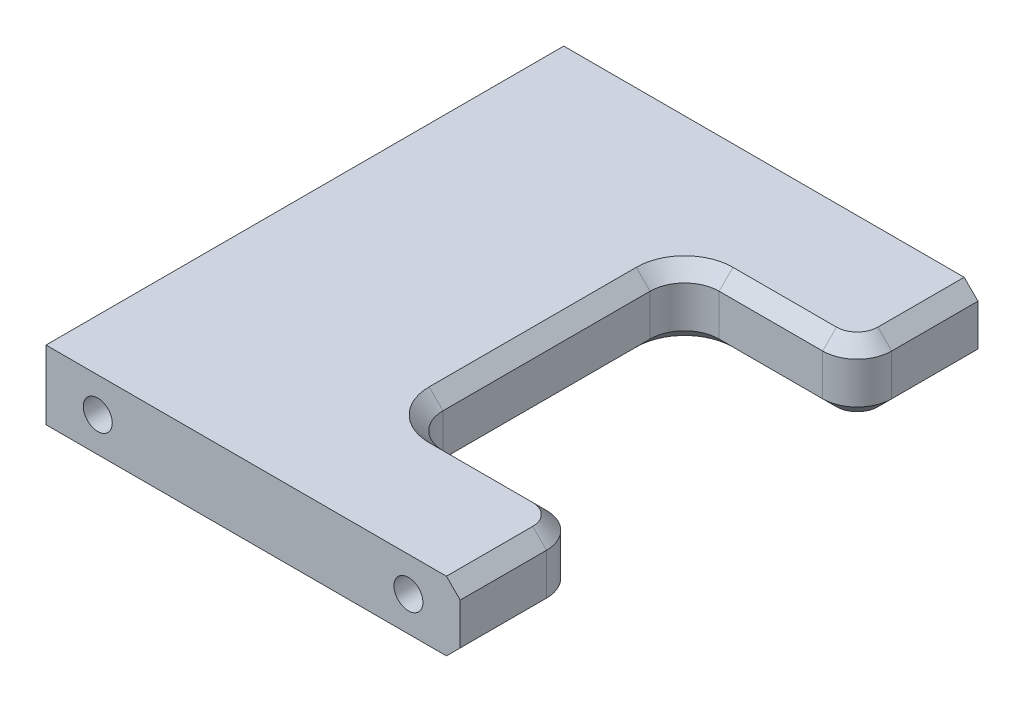
from build123d import *

# Parameters (mm, degrees)
SKETCH1_W             = 60
SKETCH1_H             = 75
BOSS_EXTRUDE1_DEPTH   = 10
M5_TAPPED_HOLE1_D     = 4.2
M5_TAPPED_HOLE1_DEPTH = 12.4
M5_TAPPED_HOLE1_TIP   = 1.2618073
M5_TAPPED_HOLE2_D     = 4.2
M5_TAPPED_HOLE2_DEPTH = 12.4
M5_TAPPED_HOLE2_TIP   = 1.2618073
SKETCH9_W             = 25
SKETCH9_H             = 40
CUT_EXTRUDE1_DEPTH    = 97.566039579
FILLET1_R             = 5
CHAMFER1_SIZE         = 2


with BuildPart() as part:
    # Sketch1 → Boss-Extrude1 (new body)
    with BuildSketch(Plane(origin=(0, 0, 0), x_dir=(1, 0, 0), z_dir=(0, 1, 0))):
        with Locations((30, 37.5)):
            Rectangle(SKETCH1_W, SKETCH1_H)
    extrude(amount=BOSS_EXTRUDE1_DEPTH)

    # M5 Tapped Hole1
    with Locations(Plane(origin=(0, 0, -75), x_dir=(-1, 0, 0), z_dir=(0, 0, -1))):
        with Locations((-7.5, 5), (-52.5, 5)):
            Hole(M5_TAPPED_HOLE1_D / 2, depth=M5_TAPPED_HOLE1_DEPTH)
            with Locations((0, 0, -(M5_TAPPED_HOLE1_DEPTH + M5_TAPPED_HOLE1_TIP / 2))):  # 118° drill point
                Cone(0, M5_TAPPED_HOLE1_D / 2, M5_TAPPED_HOLE1_TIP, mode=Mode.SUBTRACT)

    # M5 Tapped Hole2
    with Locations(Plane.XY):
        with Locations((52.5, 5), (7.5, 5)):
            Hole(M5_TAPPED_HOLE2_D / 2, depth=M5_TAPPED_HOLE2_DEPTH)
            with Locations((0, 0, -(M5_TAPPED_HOLE2_DEPTH + M5_TAPPED_HOLE2_TIP / 2))):  # 118° drill point
                Cone(0, M5_TAPPED_HOLE2_D / 2, M5_TAPPED_HOLE2_TIP, mode=Mode.SUBTRACT)

    # Sketch9 → Cut-Extrude1 (cut, through all)
    with BuildSketch(Plane(origin=(0, 10, 0), x_dir=(1, 0, 0), z_dir=(0, 1, 0))):
        with Locations((47.5, 37.5)):
            Rectangle(SKETCH9_W, SKETCH9_H)
    extrude(amount=-CUT_EXTRUDE1_DEPTH, mode=Mode.SUBTRACT)

    # Fillet1
    fillet1_edges = [part.edges().sort_by_distance(p)[0] for p in [
        (35, 5, -17.5),
        (35, 5, -57.5),
        (60, 5, -57.5),
        (60, 5, -17.5),
    ]]
    fillet(fillet1_edges, radius=FILLET1_R)

    # Chamfer1
    chamfer1_edges = [part.edges().sort_by_distance(p)[0] for p in [
        (60, 10, -6.25),
        (47.5, 10, -57.5),
        (47.5, 0, -57.5),
        (35, 10, -37.5),
        (60, 10, -68.75),
        (60, 0, -6.25),
        (47.5, 10, -17.5),
        (58.535533906, 10, -16.035533906),
        (58.535533906, 10, -58.964466094),
        (60, 0, -68.75),
        (35, 0, -37.5),
        (47.5, 0, -17.5),
        (58.535533906, 0, -16.035533906),
        (58.535533906, 0, -58.964466094),
        (36.464466094, 10, -18.964466094),
        (36.464466094, 0, -18.964466094),
        (36.464466094, 10, -56.035533906),
        (36.464466094, 0, -56.035533906),
    ]]
    chamfer(chamfer1_edges, length=CHAMFER1_SIZE)


solid = part.part
